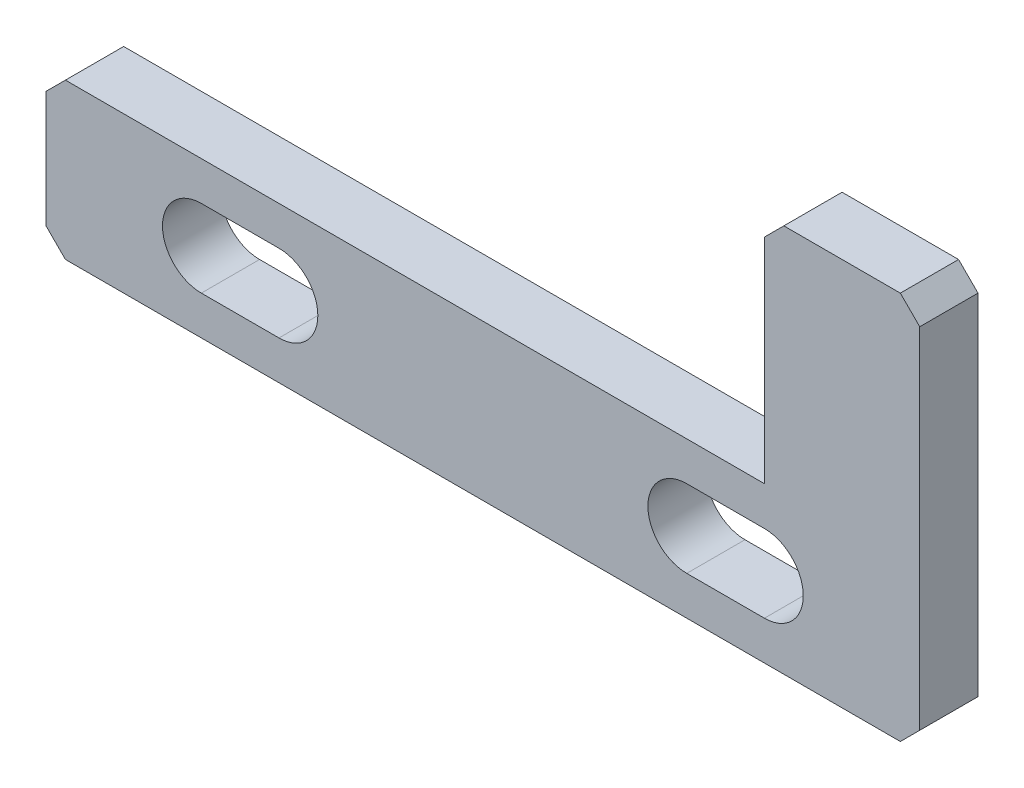
SolidWorks part; units mm, degrees
ref_plane "Front Plane" through (0, 0, 0) normal (0, 0, 1) x (1, 0, 0)
ref_plane "Top Plane" through (0, 0, 0) normal (0, 1, 0) x (1, 0, 0)
ref_plane "Right Plane" through (0, 0, 0) normal (1, 0, 0) x (0, 0, -1)
sketch "Sketch1" plane through (0, 0, 0) normal (0, 0, 1) x (1, 0, 0)
  line L0 (0, 0) -> (45, 0)
  line L1 (45, 0) -> (45, 20)
  line L2 (45, 20) -> (37, 20)
  line L3 (37, 20) -> (37, 8)
  line L4 (37, 8) -> (0, 8)
  line L5 (0, 8) -> (0, 0)
  dimension "D1" = 45
  dimension "D2" = 8
  dimension "D3" = 12
  dimension "D4" = 8
extrude "Boss-Extrude1" add sketch "Sketch1" along normal blind 3
sketch "Sketch2" plane through (0, 0, 0) normal (0, 0, -1) x (-1, 0, 0)
  line L0 (-37, 4) -> (-33, 4) construction
  line L1 (-37, 6) -> (-33, 6)
  line L2 (-37, 2) -> (-33, 2)
  line L3 (-12, 4) -> (-8, 4) construction
  line L4 (-12, 6) -> (-8, 6)
  line L5 (-12, 2) -> (-8, 2)
  line L6 (-45, 0) -> (-45, 20) construction
  line L7 (0, 0) -> (-45, 0) construction
  arc A0 (-37, 6) -> (-37, 2) centre (-37, 4) ccw
  arc A1 (-33, 2) -> (-33, 6) centre (-33, 4) ccw
  arc A2 (-12, 6) -> (-12, 2) centre (-12, 4) ccw
  arc A3 (-8, 2) -> (-8, 6) centre (-8, 4) ccw
  point P2 (-35, 4)
  point P7 (-10, 4)
  dimension "D1" = 4
  dimension "D2" = 25
  dimension "D3" = 10
  dimension "D4" = 4
  dimension "D5" = 4
extrude "Cut-Extrude1" cut sketch "Sketch2" against normal blind 3
chamfer "Chamfer1" distance 1 angle 45 5 edges at (0, 0, 1.5) (0, 8, 1.5) (37, 20, 1.5) (45, 0, 1.5) (45, 20, 1.5)
